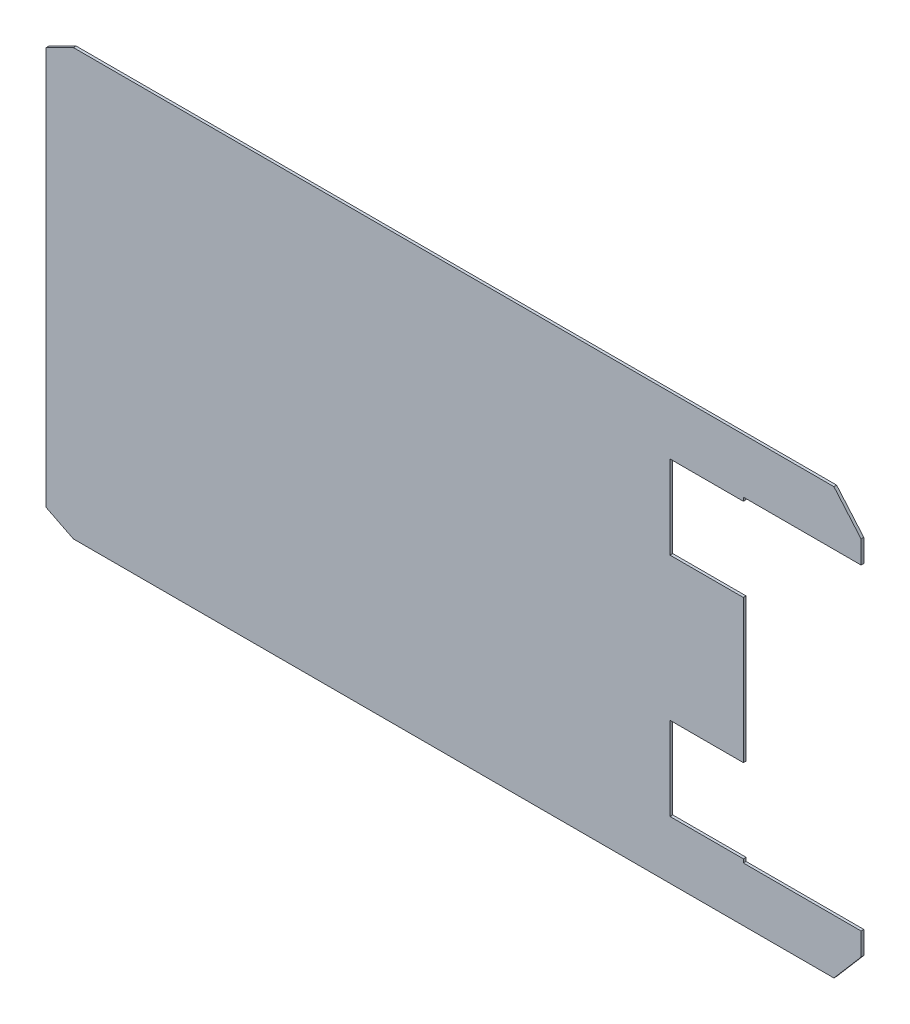
SolidWorks part; units mm, degrees
ref_plane "前视基准面" through (0, 0, 0) normal (0, 0, 1) x (1, 0, 0)
ref_plane "上视基准面" through (0, 0, 0) normal (0, 1, 0) x (1, 0, 0)
ref_plane "右视基准面" through (0, 0, 0) normal (1, 0, 0) x (0, 0, -1)
other "Configuration Table"
sketch "草图1" plane through (0, 0, 0) normal (0, 0, 1) x (1, 0, 0)
  line L0 (-620, -220) -> (-590, -235)
  line L1 (-590, -235) -> (250, -235)
  line L2 (250, -235) -> (280, -200)
  line L3 (280, -200) -> (280, -175)
  line L4 (280, -175) -> (150, -175)
  line L5 (150, -175) -> (150, 175)
  line L6 (150, 175) -> (280, 175)
  line L7 (280, 175) -> (280, 200)
  line L8 (280, 200) -> (250, 235)
  line L9 (250, 235) -> (-590, 235)
  line L10 (-590, 235) -> (-620, 220)
  line L11 (-620, 220) -> (-620, -220)
  point P0 (0, 0)
  dimension "D1" = 30
  dimension "D2" = 130
  dimension "D3" = 280
  dimension "D4" = 870
  dimension "D5" = 900
  dimension "D6" = 15
  dimension "D7" = 35
  dimension "D8" = 60
  dimension "D9" = 235
  dimension "D10" = 410
  dimension "D11" = 435
  dimension "D12" = 455
  dimension "D13" = 470
extrude "凸台-拉伸1" add sketch "草图1" against normal mid plane 3
sketch "草图2" plane through (0, 0, 0) normal (0, 0, 1) x (1, 0, 0)
  line L0 (69, 79) -> (171, 79)
  line L1 (171, 79) -> (171, 171)
  line L2 (171, 171) -> (69, 171)
  line L3 (69, 171) -> (69, 79)
  line L4 (69, -171) -> (171, -171)
  line L5 (171, -171) -> (171, -79)
  line L6 (171, -79) -> (69, -79)
  line L7 (69, -79) -> (69, -171)
  point P0 (0, 0)
  dimension "D1" = 102
  dimension "D2" = 171
  dimension "D3" = 92
  dimension "D4" = 171
  dimension "D5" = 250
  dimension "D6" = 342
extrude "切除-拉伸1" cut sketch "草图2" against normal mid plane 30
